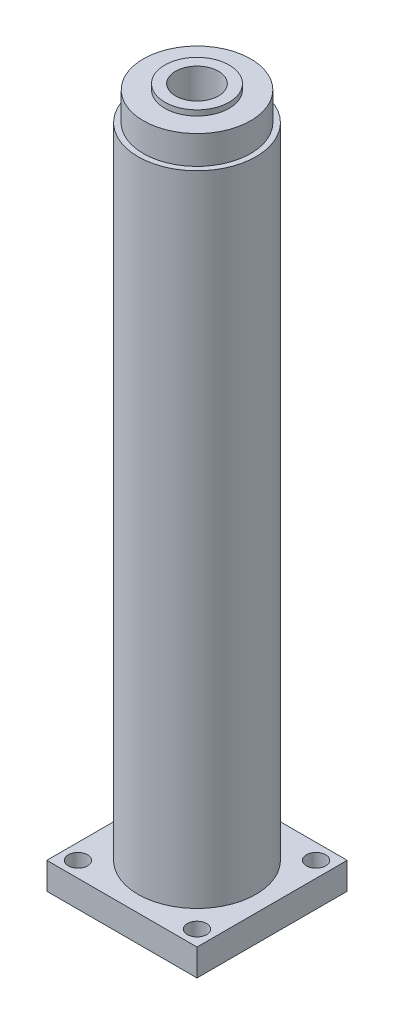
SolidWorks part; units mm, degrees
material "Q235B"
ref_plane "Front Plane" through (0, 0, 0) normal (0, 0, 1) x (1, 0, 0)
ref_plane "Top Plane" through (0, 0, 0) normal (0, 1, 0) x (1, 0, 0)
ref_plane "Right Plane" through (0, 0, 0) normal (1, 0, 0) x (0, 0, -1)
sketch "Sketch1" plane through (0, 0, 0) normal (0, 1, 0) x (1, 0, 0)
  line L1 (70, -70) -> (-70, -70)
  line L2 (70, -70) -> (70, 70)
  line L3 (70, 70) -> (-70, 70)
  line L4 (-70, -70) -> (-70, 70)
  line L5 (70, -70) -> (-70, 70) construction
  line L6 (70, 70) -> (-70, -70) construction
  circle A0 centre (-55.5, 55.5) radius 9
  circle A1 centre (55.5, 55.5) radius 9
  circle A2 centre (55.5, -55.5) radius 9
  circle A3 centre (-55.5, -55.5) radius 9
  point P0 (0, 0)
  point P17 (0, 0)
  dimension "D2" = 18
  dimension "D4" = 111
  dimension "D1" = 140
  dimension "D3" = 4
extrude "Boss-Extrude1" add sketch "Sketch1" along normal blind 25
sketch "Sketch2" plane through (0, 0, 0) normal (0, 1, 0) x (1, 0, 0)
  circle A0 centre (0, 0) radius 55
  dimension "D1" = 110
extrude "Boss-Extrude2" add sketch "Sketch2" along normal blind 652
sketch "Sketch3" plane through (0, 652, 0) normal (0, 1, 0) x (1, 0, 0)
  circle A0 centre (0, 0) radius 20
  dimension "D1" = 40
extrude "Cut-Extrude1" cut sketch "Sketch3" against normal blind 1580
sketch "Sketch4" plane through (0, 652, 0) normal (0, 1, 0) x (1, 0, 0)
  circle A1 centre (0, 0) radius 30
  dimension "D1" = 60
extrude "Cut-Extrude2" cut sketch "Sketch4" against normal blind 5 flip side to cut
sketch "Sketch6" plane through (0, 652, 0) normal (0, 1, 0) x (1, 0, 0)
  circle A0 centre (0, 0) radius 50
  dimension "D1" = 100
extrude "Cut-Extrude3" cut sketch "Sketch6" against normal blind 31.5 flip side to cut
